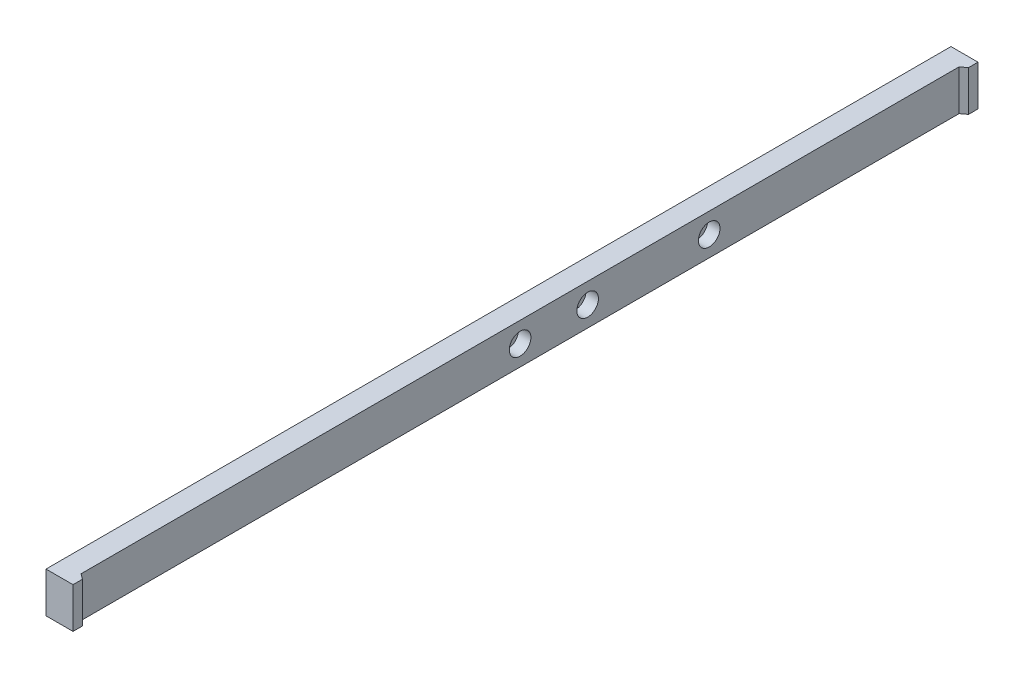
from build123d import *

# Parameters (mm, degrees)
SKETCH1_W                                            = 335
SKETCH1_H                                            = 15
BOSS_EXTRUDE1_DEPTH                                  = 10
CUT_EXTRUDE2_DEPTH                                   = 169.467355888
CBORE_FOR_M4_HEXAGON_SOCKET_HEAD_CAP_SCR_D           = 4.5
CBORE_FOR_M4_HEXAGON_SOCKET_HEAD_CAP_SCR_CBORE_D     = 8
CBORE_FOR_M4_HEXAGON_SOCKET_HEAD_CAP_SCR_CBORE_DEPTH = 4.6


with BuildPart() as part:
    # Sketch1 → Boss-Extrude1 (new body)
    with BuildSketch(Plane(origin=(0, 0, 0), x_dir=(0, 0, -1), z_dir=(1, 0, 0))):
        Rectangle(SKETCH1_W, SKETCH1_H)
    extrude(amount=BOSS_EXTRUDE1_DEPTH)

    # Sketch2 → Cut-Extrude2 (cut, through all)
    with BuildSketch(Plane.XZ.offset(7.5)):
        Polygon((8, 162.5), (8, -162.5), (10, -164), (10, 0), (10, 164), align=None)
    extrude(amount=-CUT_EXTRUDE2_DEPTH, mode=Mode.SUBTRACT)

    # CBORE for M4 Hexagon socket head cap screws1 (through all)
    with Locations(Plane(origin=(8, 0, 0), x_dir=(0, 0, -1), z_dir=(1, 0, 0))):
        with Locations((0, 0), (70, 0), (25, 0)):
            CounterBoreHole(CBORE_FOR_M4_HEXAGON_SOCKET_HEAD_CAP_SCR_D / 2, CBORE_FOR_M4_HEXAGON_SOCKET_HEAD_CAP_SCR_CBORE_D / 2, CBORE_FOR_M4_HEXAGON_SOCKET_HEAD_CAP_SCR_CBORE_DEPTH)


solid = part.part
